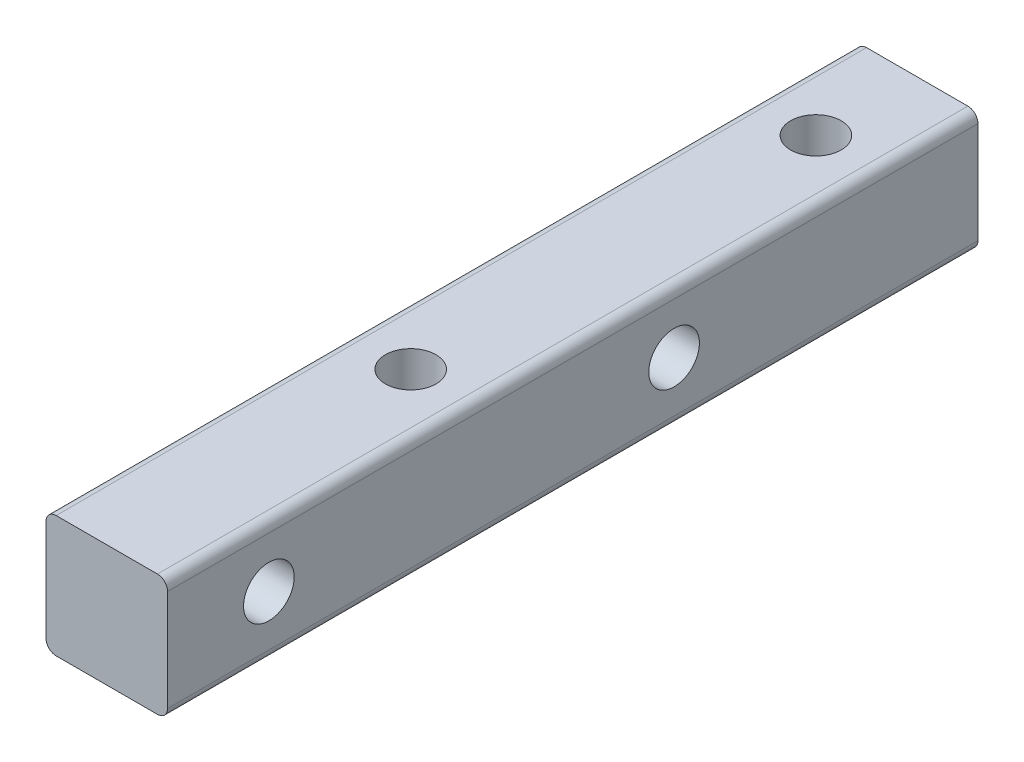
from build123d import *

# Parameters (mm, degrees)
SKETCH_1_W         = 6
SKETCH_1_H         = 6
EXTRUDE_1_DEPTH    = 20
HOLE_WIZARD_M3_1_D = 2.5
HOLE_WIZARD_M3_2_D = 2.5
FILLET_1_R         = 0.5


with BuildPart() as part:
    # 草图1 → 凸台-拉伸1 (new, symmetric)
    with BuildSketch(Plane.XY):
        Rectangle(SKETCH_1_W, SKETCH_1_H)
    extrude(amount=EXTRUDE_1_DEPTH, both=True)

    # M3 螺纹孔1 (through all)
    with Locations(Plane(origin=(0, 3, 0), x_dir=(1, 0, 0), z_dir=(0, 1, 0))):
        with Locations((0, 15), (0, -5)):
            Hole(HOLE_WIZARD_M3_1_D / 2)

    # M3 螺纹孔2 (through all)
    with Locations(Plane(origin=(3, 0, 0), x_dir=(0, 0, -1), z_dir=(1, 0, 0))):
        with Locations((-15, 0), (5, 0)):
            Hole(HOLE_WIZARD_M3_2_D / 2)

    # 圆角1
    fillet_1_edges = [part.edges().sort_by_distance(p)[0] for p in [
        (3, -3, 0),
        (-3, -3, 0),
        (-3, 3, 0),
        (3, 3, 0),
    ]]
    fillet(fillet_1_edges, radius=FILLET_1_R)


solid = part.part
